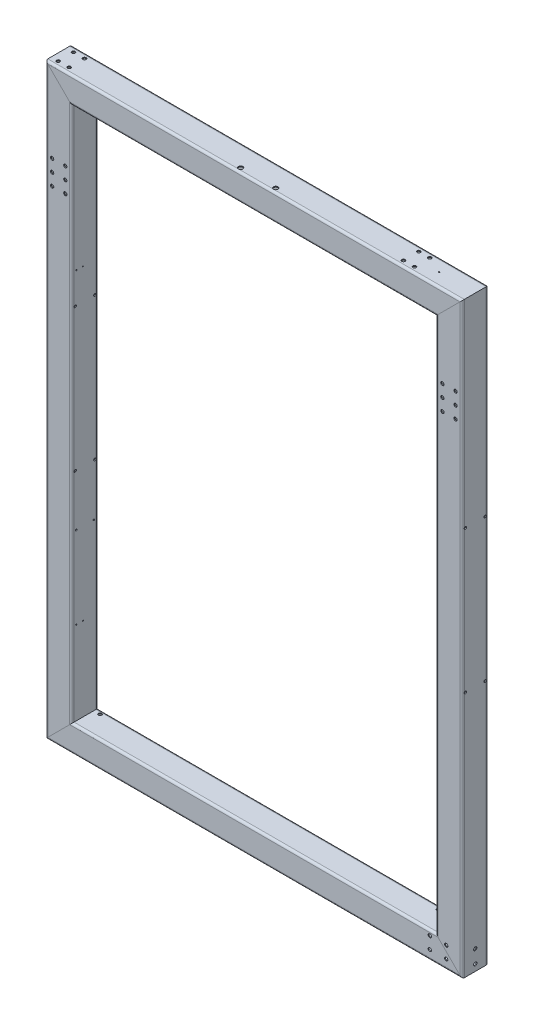
from build123d import *

# Parameters (mm, degrees)
RECTANGULAR_TUBE_120_X_80_X_8_1_DEPTH      = 1865.852813742
RECTANGULAR_TUBE_120_X_80_X_8_1_DEPTH_BACK = 85.852813742
RECTANGULAR_TUBE_120_X_80_X_8_1_2_DEPTH    = 2731.705627485
RECTANGULAR_TUBE_120_X_80_X_8_1_3_DEPTH    = 1951.705627485
RECTANGULAR_TUBE_120_X_80_X_8_1_4_DEPTH    = 2731.705627485
SKETCH4_R                                  = 7.5
SKETCH4_R_2                                = 1.5
CUT_EXTRUDE1_DEPTH                         = 10
SKETCH7_R                                  = 7.5
CUT_EXTRUDE2_DEPTH                         = 219
SKETCH6_R                                  = 5.5
SKETCH6_R_2                                = 2
CUT_EXTRUDE4_DEPTH                         = 10
M6_TAPPED_HOLE1_AT_2_COUNT                 = 2
M6_TAPPED_HOLE1_AT_2_PITCH                 = 195.576072156
M6_TAPPED_HOLE1_AT_3_COUNT                 = 2
M6_TAPPED_HOLE1_AT_3_PITCH                 = 200.124960962
M6_TAPPED_HOLE1_AT_4_COUNT                 = 2
M6_TAPPED_HOLE1_AT_4_PITCH                 = 1215.092589065
M6_TAPPED_HOLE1_AT_5_COUNT                 = 2
M6_TAPPED_HOLE1_AT_5_PITCH                 = 1215.83304775
SKETCH22_R                                 = 5.5
SKETCH22_R_2                               = 7.5
CUT_EXTRUDE5_DEPTH                         = 10
SKETCH33_R                                 = 7.5
CUT_EXTRUDE9_DEPTH                         = 10
SKETCH34_R                                 = 10
SKETCH34_R_2                               = 7.5
CUT_EXTRUDE10_DEPTH                        = 10
M8_TAPPED_HOLE5_AT_2_COUNT                 = 2
M8_TAPPED_HOLE5_AT_2_PITCH                 = 80
M6_TAPPED_HOLE4_AT_2_COUNT                 = 2
M6_TAPPED_HOLE4_AT_2_PITCH                 = 30
M6_TAPPED_HOLE4_AT_3_COUNT                 = 2
M6_TAPPED_HOLE4_AT_3_PITCH                 = 1400
M6_TAPPED_HOLE4_AT_4_COUNT                 = 2
M6_TAPPED_HOLE4_AT_4_PITCH                 = 1400.321391681
M6_TAPPED_HOLE5_AT_2_COUNT                 = 2
M6_TAPPED_HOLE5_AT_2_PITCH                 = 30
M6_TAPPED_HOLE5_AT_3_COUNT                 = 2
M6_TAPPED_HOLE5_AT_3_PITCH                 = 1400
M6_TAPPED_HOLE5_AT_4_COUNT                 = 2
M6_TAPPED_HOLE5_AT_4_PITCH                 = 1400.321391681
M8_TAPPED_HOLE6_AT_2_COUNT                 = 2
M8_TAPPED_HOLE6_AT_2_PITCH                 = 80
SKETCH44_R                                 = 5.5
CUT_EXTRUDE11_DEPTH                        = 10
SKETCH45_R                                 = 7.5
CUT_EXTRUDE12_DEPTH                        = 10


with BuildPart() as part:
    # Sketch11 → Rectangular Tube 120 X 80 X 8(1) (new, two sides: drawn at the far end of the back side and taken through both)
    with BuildSketch(Plane(origin=(-890, 1280, 0), x_dir=(0, 0, -1), z_dir=(1, 0, 0)).offset(-RECTANGULAR_TUBE_120_X_80_X_8_1_DEPTH_BACK)):
        with BuildLine():
            Line((-50, -60), (50, -60))
            ThreePointArc((50, -60), (57.071067812, -57.071067812), (60, -50))
            Line((60, -50), (60, 50))
            ThreePointArc((60, 50), (57.071067812, 57.071067812), (50, 60))
            Line((50, 60), (-50, 60))
            ThreePointArc((-50, 60), (-57.071067812, 57.071067812), (-60, 50))
            Line((-60, 50), (-60, -50))
            ThreePointArc((-60, -50), (-57.071067812, -57.071067812), (-50, -60))
        make_face()
        with BuildLine():
            Line((-50, -56), (50, -56))
            ThreePointArc((50, -56), (54.242640687, -54.242640687), (56, -50))
            Line((56, -50), (56, 50))
            ThreePointArc((56, 50), (54.242640687, 54.242640687), (50, 56))
            Line((50, 56), (-50, 56))
            ThreePointArc((-50, 56), (-54.242640687, 54.242640687), (-56, 50))
            Line((-56, 50), (-56, -50))
            ThreePointArc((-56, -50), (-54.242640687, -54.242640687), (-50, -56))
        make_face(mode=Mode.SUBTRACT)
    extrude(amount=RECTANGULAR_TUBE_120_X_80_X_8_1_DEPTH + RECTANGULAR_TUBE_120_X_80_X_8_1_DEPTH_BACK)

    # Rectangular Tube 120 X 80 X 8(1) mitre 1
    split(bisect_by=Plane(origin=(-890, 1280, 0), x_dir=(-0.707106781, 0.707106781, 0), z_dir=(0.707106781, 0.707106781, 0)), keep=Keep.TOP)

    # Rectangular Tube 120 X 80 X 8(1) mitre 2
    split(bisect_by=Plane(origin=(890, 1280, 0), x_dir=(-0.707106781, -0.707106781, 0), z_dir=(-0.707106781, 0.707106781, 0)), keep=Keep.TOP)


with BuildPart() as body_2:
    # Sketch11 on segment 2 (carried to segment 2) → Rectangular Tube 120 X 80 X 8_1 2 (new body)
    with BuildSketch(Plane(origin=(890, 1365.852813742, 0), x_dir=(0, 0, -1), z_dir=(0, -1, 0))):
        with BuildLine():
            Line((-50, -60), (50, -60))
            ThreePointArc((50, -60), (57.071067812, -57.071067812), (60, -50))
            Line((60, -50), (60, 50))
            ThreePointArc((60, 50), (57.071067812, 57.071067812), (50, 60))
            Line((50, 60), (-50, 60))
            ThreePointArc((-50, 60), (-57.071067812, 57.071067812), (-60, 50))
            Line((-60, 50), (-60, -50))
            ThreePointArc((-60, -50), (-57.071067812, -57.071067812), (-50, -60))
        make_face()
        with BuildLine():
            Line((-50, -56), (50, -56))
            ThreePointArc((50, -56), (54.242640687, -54.242640687), (56, -50))
            Line((56, -50), (56, 50))
            ThreePointArc((56, 50), (54.242640687, 54.242640687), (50, 56))
            Line((50, 56), (-50, 56))
            ThreePointArc((-50, 56), (-54.242640687, 54.242640687), (-56, 50))
            Line((-56, 50), (-56, -50))
            ThreePointArc((-56, -50), (-54.242640687, -54.242640687), (-50, -56))
        make_face(mode=Mode.SUBTRACT)
    extrude(amount=RECTANGULAR_TUBE_120_X_80_X_8_1_2_DEPTH)

    # Rectangular Tube 120 X 80 X 8_1 2 mitre
    split(bisect_by=Plane(origin=(890, 1280, 0), x_dir=(0.707106781, 0.707106781, 0), z_dir=(0.707106781, -0.707106781, 0)), keep=Keep.TOP)

    # Rectangular Tube 120 X 80 X 8_1 2 mi 2
    split(bisect_by=Plane(origin=(890, -1280, 0), x_dir=(-0.707106781, 0.707106781, 0), z_dir=(0.707106781, 0.707106781, 0)), keep=Keep.TOP)


with BuildPart() as body_3:
    # Sketch11 on segment 3 (carried to segment 3) → Rectangular Tube 120 X 80 X 8_1 3 (new body)
    with BuildSketch(Plane(origin=(975.852813742, -1280, 0), x_dir=(0, 0, -1), z_dir=(-1, 0, 0))):
        with BuildLine():
            Line((-50, -60), (50, -60))
            ThreePointArc((50, -60), (57.071067812, -57.071067812), (60, -50))
            Line((60, -50), (60, 50))
            ThreePointArc((60, 50), (57.071067812, 57.071067812), (50, 60))
            Line((50, 60), (-50, 60))
            ThreePointArc((-50, 60), (-57.071067812, 57.071067812), (-60, 50))
            Line((-60, 50), (-60, -50))
            ThreePointArc((-60, -50), (-57.071067812, -57.071067812), (-50, -60))
        make_face()
        with BuildLine():
            Line((-50, -56), (50, -56))
            ThreePointArc((50, -56), (54.242640687, -54.242640687), (56, -50))
            Line((56, -50), (56, 50))
            ThreePointArc((56, 50), (54.242640687, 54.242640687), (50, 56))
            Line((50, 56), (-50, 56))
            ThreePointArc((-50, 56), (-54.242640687, 54.242640687), (-56, 50))
            Line((-56, 50), (-56, -50))
            ThreePointArc((-56, -50), (-54.242640687, -54.242640687), (-50, -56))
        make_face(mode=Mode.SUBTRACT)
    extrude(amount=RECTANGULAR_TUBE_120_X_80_X_8_1_3_DEPTH)

    # Rectangular Tube 120 X 80 X 8_1 3 mitre
    split(bisect_by=Plane(origin=(-890, -1280, 0), x_dir=(0.707106781, 0.707106781, 0), z_dir=(0.707106781, -0.707106781, 0)), keep=Keep.TOP)

    # Rectangular Tube 120 X 80 X 8_1 3 mi 2
    split(bisect_by=Plane(origin=(890, -1280, 0), x_dir=(0.707106781, -0.707106781, 0), z_dir=(-0.707106781, -0.707106781, 0)), keep=Keep.TOP)

    # Sketch33 → Cut-Extrude9 (cut)
    with BuildSketch(Plane(origin=(0, -1220, 0), x_dir=(1, 0, 0), z_dir=(0, 1, 0))):
        with Locations(Location((741.5, 40, 0), (0, 0, 270))):
            Circle(SKETCH33_R)
        with Locations(Location((-801.5, 40, 0), (0, 0, 270))):
            Circle(SKETCH33_R)
    extrude(amount=-CUT_EXTRUDE9_DEPTH, mode=Mode.SUBTRACT)


with BuildPart() as body_4:
    # Sketch11 on segment 4 (carried to segment 4) → Rectangular Tube 120 X 80 X 8_1 4 (new body)
    with BuildSketch(Plane(origin=(-890, -1365.852813742, 0), x_dir=(0, 0, -1), z_dir=(0, 1, 0))):
        with BuildLine():
            Line((-50, -60), (50, -60))
            ThreePointArc((50, -60), (57.071067812, -57.071067812), (60, -50))
            Line((60, -50), (60, 50))
            ThreePointArc((60, 50), (57.071067812, 57.071067812), (50, 60))
            Line((50, 60), (-50, 60))
            ThreePointArc((-50, 60), (-57.071067812, 57.071067812), (-60, 50))
            Line((-60, 50), (-60, -50))
            ThreePointArc((-60, -50), (-57.071067812, -57.071067812), (-50, -60))
        make_face()
        with BuildLine():
            Line((-50, -56), (50, -56))
            ThreePointArc((50, -56), (54.242640687, -54.242640687), (56, -50))
            Line((56, -50), (56, 50))
            ThreePointArc((56, 50), (54.242640687, 54.242640687), (50, 56))
            Line((50, 56), (-50, 56))
            ThreePointArc((-50, 56), (-54.242640687, 54.242640687), (-56, 50))
            Line((-56, 50), (-56, -50))
            ThreePointArc((-56, -50), (-54.242640687, -54.242640687), (-50, -56))
        make_face(mode=Mode.SUBTRACT)
    extrude(amount=RECTANGULAR_TUBE_120_X_80_X_8_1_4_DEPTH)

    # Rectangular Tube 120 X 80 X 8_1 4 mitre
    split(bisect_by=Plane(origin=(-890, 1280, 0), x_dir=(0.707106781, -0.707106781, 0), z_dir=(-0.707106781, -0.707106781, 0)), keep=Keep.TOP)

    # Rectangular Tube 120 X 80 X 8_1 4 mi 2
    split(bisect_by=Plane(origin=(-890, -1280, 0), x_dir=(-0.707106781, -0.707106781, 0), z_dir=(-0.707106781, 0.707106781, 0)), keep=Keep.TOP)


with BuildPart() as cut_extrude1_tool:
    # Sketch4 → Cut-Extrude1 (new body)
    with BuildSketch(Plane(origin=(0, 0, -60), x_dir=(-1, 0, 0), z_dir=(0, 0, -1))):
        with Locations((-80, 1298)):
            Circle(SKETCH4_R)
        with Locations((-80, 1278)):
            Circle(SKETCH4_R)
        with Locations((-125, 1270)):
            Circle(SKETCH4_R)
        with Locations((80, 1298)):
            Circle(SKETCH4_R)
        with Locations((80, 1278)):
            Circle(SKETCH4_R)
        with Locations((125, 1270)):
            Circle(SKETCH4_R)
        with Locations((-920, 967)):
            Circle(SKETCH4_R)
        with Locations((-860, 967)):
            Circle(SKETCH4_R)
        with Locations((-920, 912)):
            Circle(SKETCH4_R)
        with Locations((-860, 912)):
            Circle(SKETCH4_R)
        with Locations((-920, 857)):
            Circle(SKETCH4_R)
        with Locations((-860, 857)):
            Circle(SKETCH4_R)
        with Locations(Location((860, 967, 0), (0, 0, 180))):
            Circle(SKETCH4_R)
        with Locations(Location((920, 967, 0), (0, 0, 180))):
            Circle(SKETCH4_R)
        with Locations(Location((860, 912, 0), (0, 0, 180))):
            Circle(SKETCH4_R)
        with Locations(Location((920, 912, 0), (0, 0, 180))):
            Circle(SKETCH4_R)
        with Locations(Location((860, 857, 0), (0, 0, 180))):
            Circle(SKETCH4_R)
        with Locations(Location((920, 857, 0), (0, 0, 180))):
            Circle(SKETCH4_R)
        with Locations((-937, 573)):
            Circle(SKETCH4_R_2)
        with Locations((-843, 573)):
            Circle(SKETCH4_R_2)
        with Locations((-937, 479)):
            Circle(SKETCH4_R_2)
        with Locations((-843, 479)):
            Circle(SKETCH4_R_2)
        with Locations(Location((843, 479, 0), (0, 0, 180))):
            Circle(SKETCH4_R_2)
        with Locations(Location((937, 479, 0), (0, 0, 180))):
            Circle(SKETCH4_R_2)
        with Locations(Location((843, 573, 0), (0, 0, 180))):
            Circle(SKETCH4_R_2)
        with Locations(Location((937, 573, 0), (0, 0, 180))):
            Circle(SKETCH4_R_2)
    extrude(amount=-CUT_EXTRUDE1_DEPTH)


with BuildPart() as part_1:
    add(part.part)

    # Cut-Extrude1: cut by cut_extrude1_tool
    add(cut_extrude1_tool.part, mode=Mode.SUBTRACT)

    # Sketch34 → Cut-Extrude10 (cut)
    with BuildSketch(Plane(origin=(0, 1340, 0), x_dir=(1, 0, 0), z_dir=(0, 1, 0))):
        with Locations(Location((-80, -40, 0), (0, 0, 270))):
            Circle(SKETCH34_R)
        with Locations(Location((80, -40, 0), (0, 0, 270))):
            Circle(SKETCH34_R)
        with Locations(Location((-917.5, -35, 0), (0, 0, 90))):
            Circle(SKETCH34_R_2)
        with Locations(Location((-917.5, 35, 0), (0, 0, 90))):
            Circle(SKETCH34_R_2)
        with Locations(Location((-867.5, 35, 0), (0, 0, 90))):
            Circle(SKETCH34_R_2)
        with Locations(Location((-867.5, -35, 0), (0, 0, 90))):
            Circle(SKETCH34_R_2)
        with Locations(Location((657.5, 35, 0), (0, 0, 90))):
            Circle(SKETCH34_R_2)
        with Locations(Location((707.5, 35, 0), (0, 0, 90))):
            Circle(SKETCH34_R_2)
        with Locations(Location((657.5, -35, 0), (0, 0, 90))):
            Circle(SKETCH34_R_2)
        with Locations(Location((707.5, -35, 0), (0, 0, 90))):
            Circle(SKETCH34_R_2)
    extrude(amount=-CUT_EXTRUDE10_DEPTH, mode=Mode.SUBTRACT)

    # Sketch48 → M6 Tapped Hole6 (revolve, cut)
    with BuildSketch(Plane(origin=(785, 1340, 0), x_dir=(0, 0, 1), z_dir=(1, 0, 0))):
        Polygon((0, 0), (0, 16.502151548), (2.5, 15), (2.5, 0), align=None)
    revolve(axis=Axis((785, 1346.35, 0), (0, -1, 0)), mode=Mode.SUBTRACT)


with BuildPart() as body_2_1:
    add(body_2.part)

    # Cut-Extrude1: cut by cut_extrude1_tool
    add(cut_extrude1_tool.part, mode=Mode.SUBTRACT)


with BuildPart() as body_4_1:
    add(body_4.part)

    # Cut-Extrude1: cut by cut_extrude1_tool
    add(cut_extrude1_tool.part, mode=Mode.SUBTRACT)


with BuildPart() as cut_extrude2_tool:
    # Sketch7 → Cut-Extrude2 (new body)
    with BuildSketch(Plane(origin=(0, 0, -60), x_dir=(-1, 0, 0), z_dir=(0, 0, -1))):
        with Locations(Location((860, 857, 0), (0, 0, 180))):
            Circle(SKETCH7_R)
        with Locations(Location((920, 857, 0), (0, 0, 180))):
            Circle(SKETCH7_R)
        with Locations(Location((920, 967, 0), (0, 0, 180))):
            Circle(SKETCH7_R)
        with Locations(Location((920, 912, 0), (0, 0, 180))):
            Circle(SKETCH7_R)
        with Locations(Location((860, 912, 0), (0, 0, 180))):
            Circle(SKETCH7_R)
        with Locations(Location((860, 967, 0), (0, 0, 180))):
            Circle(SKETCH7_R)
        with Locations((-860, 857)):
            Circle(SKETCH7_R)
        with Locations((-920, 857)):
            Circle(SKETCH7_R)
        with Locations((-860, 912)):
            Circle(SKETCH7_R)
        with Locations((-860, 967)):
            Circle(SKETCH7_R)
        with Locations((-920, 912)):
            Circle(SKETCH7_R)
        with Locations((-920, 967)):
            Circle(SKETCH7_R)
    extrude(amount=-CUT_EXTRUDE2_DEPTH)


with BuildPart() as body_2_2:
    add(body_2_1.part)

    # Cut-Extrude2: cut by cut_extrude2_tool
    add(cut_extrude2_tool.part, mode=Mode.SUBTRACT)

    # Sketch22 → Cut-Extrude5 (cut)
    with BuildSketch(Plane(origin=(950, 0, 0), x_dir=(0, 0, -1), z_dir=(1, 0, 0))):
        with Locations(Location((-45, 435, 0), (0, 0, 155.380022671))):
            Circle(SKETCH22_R)
        with Locations(Location((45, 435, 0), (0, 0, 24.619977329))):
            Circle(SKETCH22_R)
        with Locations(Location((-45, -215, 0), (0, 0, 155.380022671))):
            Circle(SKETCH22_R)
        with Locations(Location((45, -215, 0), (0, 0, 24.619977329))):
            Circle(SKETCH22_R)
        with Locations((0, -1250)):
            Circle(SKETCH22_R_2)
        with Locations((0, -1310)):
            Circle(SKETCH22_R_2)
    extrude(amount=-CUT_EXTRUDE5_DEPTH, mode=Mode.SUBTRACT)

    # Sketch41 → M6 Tapped Hole5 (revolve, cut)
    with BuildSketch(Plane(origin=(830, 560, 10), x_dir=(0, 0, 1), z_dir=(0, 1, 0))):
        Polygon((0, 0), (0, 16.502151548), (2.5, 15), (2.5, 0), align=None)
    m6_tapped_hole5 = revolve(axis=Axis((823.65, 560, 10), (1, 0, 0)), mode=Mode.SUBTRACT)

    # M6 Tapped Hole5 at 2: M6 Tapped Hole5 ×2
    with Locations(*[(0, 0, i * M6_TAPPED_HOLE5_AT_2_PITCH) for i in range(1, M6_TAPPED_HOLE5_AT_2_COUNT)]):
        add(m6_tapped_hole5, mode=Mode.SUBTRACT)

    # M6 Tapped Hole5 at 3: M6 Tapped Hole5 ×2
    with Locations(*[(0, -i * M6_TAPPED_HOLE5_AT_3_PITCH, 0) for i in range(1, M6_TAPPED_HOLE5_AT_3_COUNT)]):
        add(m6_tapped_hole5, mode=Mode.SUBTRACT)

    # M6 Tapped Hole5 at 4: M6 Tapped Hole5 ×2
    with Locations(*[Vector(0, -0.9997704872016389, 0.02142365329717798) * (i * M6_TAPPED_HOLE5_AT_4_PITCH) for i in range(1, M6_TAPPED_HOLE5_AT_4_COUNT)]):
        add(m6_tapped_hole5, mode=Mode.SUBTRACT)

    # Sketch43 → M8 Tapped Hole6 (revolve, cut)
    with BuildSketch(Plane(origin=(830, -466, -40), x_dir=(0, 0, 1), z_dir=(0, 1, 0))):
        Polygon((0, 0), (0, 21.792926105), (3.4, 19.75), (3.4, 0), align=None)
    m8_tapped_hole6 = revolve(axis=Axis((823.65, -466, -40), (1, 0, 0)), mode=Mode.SUBTRACT)

    # M8 Tapped Hole6 at 2: M8 Tapped Hole6 ×2
    with Locations(*[(0, 0, i * M8_TAPPED_HOLE6_AT_2_PITCH) for i in range(1, M8_TAPPED_HOLE6_AT_2_COUNT)]):
        add(m8_tapped_hole6, mode=Mode.SUBTRACT)


with BuildPart() as body_4_2:
    add(body_4_1.part)

    # Cut-Extrude2: cut by cut_extrude2_tool
    add(cut_extrude2_tool.part, mode=Mode.SUBTRACT)

    # Sketch6 → Cut-Extrude4 (cut)
    with BuildSketch(Plane.ZY.offset(950)):
        with Locations((-32.5, 1065)):
            Circle(SKETCH6_R)
        with Locations((32.5, 1065)):
            Circle(SKETCH6_R)
        with Locations((-32.5, 630)):
            Circle(SKETCH6_R)
        with Locations((32.5, 630)):
            Circle(SKETCH6_R)
        with Locations((15, 225)):
            Circle(SKETCH6_R_2)
        with Locations((45, 225)):
            Circle(SKETCH6_R_2)
        with Locations((15, -795)):
            Circle(SKETCH6_R_2)
        with Locations((45, -795)):
            Circle(SKETCH6_R_2)
        with Locations((0, 420)):
            Circle(SKETCH6_R_2)
    extrude(amount=-CUT_EXTRUDE4_DEPTH, mode=Mode.SUBTRACT)

    # Sketch14 → M6 Tapped Hole1 (revolve, cut)
    with BuildSketch(Plane(origin=(-950, 420, 0), x_dir=(0, 0, 1), z_dir=(0, 1, 0))):
        Polygon((0, 0), (0, 16.502151548), (2.5, 15), (2.5, 0), align=None)
    m6_tapped_hole1 = revolve(axis=Axis((-956.35, 420, 0), (1, 0, 0)), mode=Mode.SUBTRACT)

    # M6 Tapped Hole1 at 2: M6 Tapped Hole1 ×2
    with Locations(*[Vector(0, -0.9970544855015816, 0.0766964988847371) * (i * M6_TAPPED_HOLE1_AT_2_PITCH) for i in range(1, M6_TAPPED_HOLE1_AT_2_COUNT)]):
        add(m6_tapped_hole1, mode=Mode.SUBTRACT)

    # M6 Tapped Hole1 at 3: M6 Tapped Hole1 ×2
    with Locations(*[Vector(0, -0.97439119569462, 0.22485950669875834) * (i * M6_TAPPED_HOLE1_AT_3_PITCH) for i in range(1, M6_TAPPED_HOLE1_AT_3_COUNT)]):
        add(m6_tapped_hole1, mode=Mode.SUBTRACT)

    # M6 Tapped Hole1 at 4: M6 Tapped Hole1 ×2
    with Locations(*[Vector(0, -0.9999238008152207, 0.012344738281669394) * (i * M6_TAPPED_HOLE1_AT_4_PITCH) for i in range(1, M6_TAPPED_HOLE1_AT_4_COUNT)]):
        add(m6_tapped_hole1, mode=Mode.SUBTRACT)

    # M6 Tapped Hole1 at 5: M6 Tapped Hole1 ×2
    with Locations(*[Vector(0, -0.9993148337667671, 0.037011660509880265) * (i * M6_TAPPED_HOLE1_AT_5_PITCH) for i in range(1, M6_TAPPED_HOLE1_AT_5_COUNT)]):
        add(m6_tapped_hole1, mode=Mode.SUBTRACT)

    # Sketch37 → M8 Tapped Hole5 (revolve, cut)
    with BuildSketch(Plane(origin=(-830, -466, 40), x_dir=(0, 0, -1), z_dir=(0, 1, 0))):
        Polygon((0, 0), (0, 21.792926105), (3.4, 19.75), (3.4, 0), align=None)
    m8_tapped_hole5 = revolve(axis=Axis((-823.65, -466, 40), (-1, 0, 0)), mode=Mode.SUBTRACT)

    # M8 Tapped Hole5 at 2: M8 Tapped Hole5 ×2
    with Locations(*[(0, 0, -i * M8_TAPPED_HOLE5_AT_2_PITCH) for i in range(1, M8_TAPPED_HOLE5_AT_2_COUNT)]):
        add(m8_tapped_hole5, mode=Mode.SUBTRACT)

    # Sketch39 → M6 Tapped Hole4 (revolve, cut)
    with BuildSketch(Plane(origin=(-830, 560, 40), x_dir=(0, 0, -1), z_dir=(0, 1, 0))):
        Polygon((0, 0), (0, 16.502151548), (2.5, 15), (2.5, 0), align=None)
    m6_tapped_hole4 = revolve(axis=Axis((-823.65, 560, 40), (-1, 0, 0)), mode=Mode.SUBTRACT)

    # M6 Tapped Hole4 at 2: M6 Tapped Hole4 ×2
    with Locations(*[(0, 0, -i * M6_TAPPED_HOLE4_AT_2_PITCH) for i in range(1, M6_TAPPED_HOLE4_AT_2_COUNT)]):
        add(m6_tapped_hole4, mode=Mode.SUBTRACT)

    # M6 Tapped Hole4 at 3: M6 Tapped Hole4 ×2
    with Locations(*[(0, -i * M6_TAPPED_HOLE4_AT_3_PITCH, 0) for i in range(1, M6_TAPPED_HOLE4_AT_3_COUNT)]):
        add(m6_tapped_hole4, mode=Mode.SUBTRACT)

    # M6 Tapped Hole4 at 4: M6 Tapped Hole4 ×2
    with Locations(*[Vector(0, -0.9997704872016389, -0.021423653297177974) * (i * M6_TAPPED_HOLE4_AT_4_PITCH) for i in range(1, M6_TAPPED_HOLE4_AT_4_COUNT)]):
        add(m6_tapped_hole4, mode=Mode.SUBTRACT)

    # Sketch44 → Cut-Extrude11 (cut)
    with BuildSketch(Plane(origin=(-830, 0, 0), x_dir=(0, 0, -1), z_dir=(1, 0, 0))):
        with Locations(Location((-45, 420, 0), (0, 0, 155.380022671))):
            Circle(SKETCH44_R)
        with Locations(Location((45, 420, 0), (0, 0, 24.619977329))):
            Circle(SKETCH44_R)
        with Locations(Location((-45, -230, 0), (0, 0, 204.619977329))):
            Circle(SKETCH44_R)
        with Locations(Location((45, -230, 0), (0, 0, 335.380022671))):
            Circle(SKETCH44_R)
    extrude(amount=-CUT_EXTRUDE11_DEPTH, mode=Mode.SUBTRACT)


with BuildPart() as cut_extrude12_tool:
    # Sketch45 → Cut-Extrude12 (new body)
    with BuildSketch(Plane.XY.offset(60)):
        with Locations((802.5, -1242.5)):
            Circle(SKETCH45_R)
        with Locations((877.5, -1242.5)):
            Circle(SKETCH45_R)
        with Locations((877.5, -1297.5)):
            Circle(SKETCH45_R)
        with Locations((802.5, -1297.5)):
            Circle(SKETCH45_R)
    extrude(amount=-CUT_EXTRUDE12_DEPTH)


with BuildPart() as body_2_3:
    add(body_2_2.part)

    # Cut-Extrude12: cut by cut_extrude12_tool
    add(cut_extrude12_tool.part, mode=Mode.SUBTRACT)


with BuildPart() as body_3_1:
    add(body_3.part)

    # Cut-Extrude12: cut by cut_extrude12_tool
    add(cut_extrude12_tool.part, mode=Mode.SUBTRACT)


solid = Compound([part_1.part, body_4_2.part, body_2_3.part, body_3_1.part])
